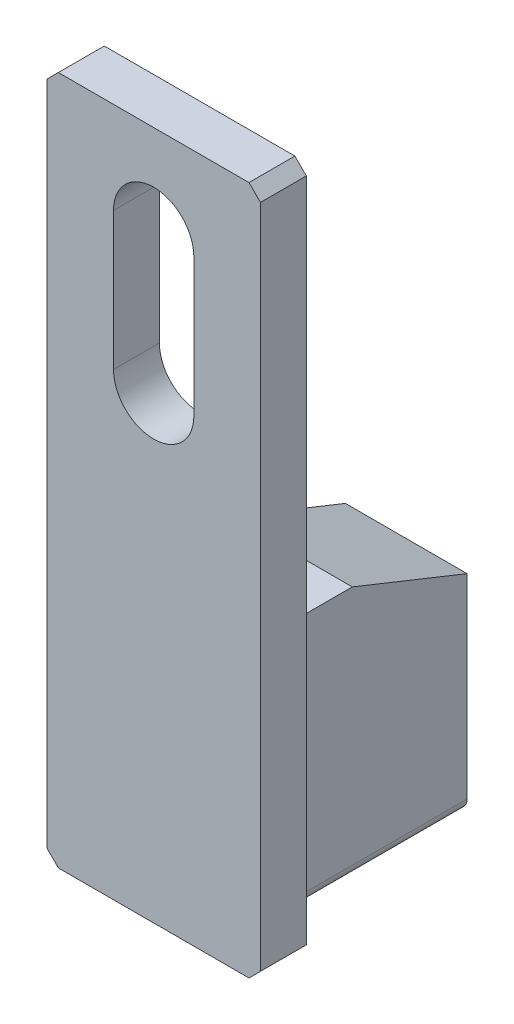
SolidWorks part; units mm, degrees
ref_plane "Front Plane" through (0, 0, 0) normal (0, 0, 1) x (1, 0, 0)
ref_plane "Top Plane" through (0, 0, 0) normal (0, 1, 0) x (1, 0, 0)
ref_plane "Right Plane" through (0, 0, 0) normal (1, 0, 0) x (0, 0, -1)
sketch "Sketch1" plane through (0, 0, 0) normal (0, 0, 1) x (1, 0, 0)
  line L1 (-2.65, 5.5) -> (2.65, 5.5)
  line L2 (-2.65, 5.5) -> (-2.65, -5.5)
  line L3 (-2.65, -5.5) -> (2.65, -5.5)
  line L4 (2.65, 5.5) -> (2.65, -5.5)
  line L5 (-2.65, 5.5) -> (2.65, -5.5) construction
  line L6 (-2.65, -5.5) -> (2.65, 5.5) construction
  point P0 (0, 0)
  dimension "D1" = 5.3
  dimension "D2" = 11
extrude "Boss-Extrude1" add sketch "Sketch1" along normal blind 9
sketch "Sketch2" plane through (0, 0, 9) normal (0, 0, 1) x (1, 0, 0)
  line L0 (2.65, -5.5) -> (2.65, 5.5) construction
  line L1 (4.65, -5.5) -> (-4.65, -5.5)
  line L2 (4.65, -5.5) -> (4.65, 24.5)
  line L3 (4.65, 24.5) -> (-4.65, 24.5)
  line L4 (-4.65, -5.5) -> (-4.65, 24.5)
  line L5 (-2.65, 5.5) -> (-2.65, -5.5) construction
  line L6 (-2.65, -5.5) -> (2.65, -5.5) construction
  dimension "D1" = 2
  dimension "D2" = 2
  dimension "D3" = 30
extrude "Boss-Extrude2" add sketch "Sketch2" along normal blind 2
sketch "Sketch3" plane through (0, 0, 11) normal (0, 0, 1) x (1, 0, 0)
  line L0 (0, 20.5) -> (0, 14.5) construction
  line L1 (1.75, 20.5) -> (1.75, 14.5)
  line L2 (-1.75, 20.5) -> (-1.75, 14.5)
  line L3 (4.65, 24.5) -> (-4.65, 24.5) construction
  arc A0 (1.75, 20.5) -> (-1.75, 20.5) centre (0, 20.5) ccw
  arc A1 (-1.75, 14.5) -> (1.75, 14.5) centre (0, 14.5) ccw
  point P3 (0, 17.5)
  dimension "D3" = 4
  dimension "D1" = 3.5
  dimension "D2" = 6
extrude "Cut-Extrude1" cut sketch "Sketch3" against normal blind 10
chamfer "Chamfer1" distance 0.5 angle 45 4 edges at (-4.65, -5.5, 10) (4.65, -5.5, 10) (4.65, 24.5, 10) (-4.65, 24.5, 10)
fillet "Fillet1" radius 0.5 2 edges
chamfer "Chamfer2" distance 2 distance2 5 1 edges at (0, 5.5, 0)
